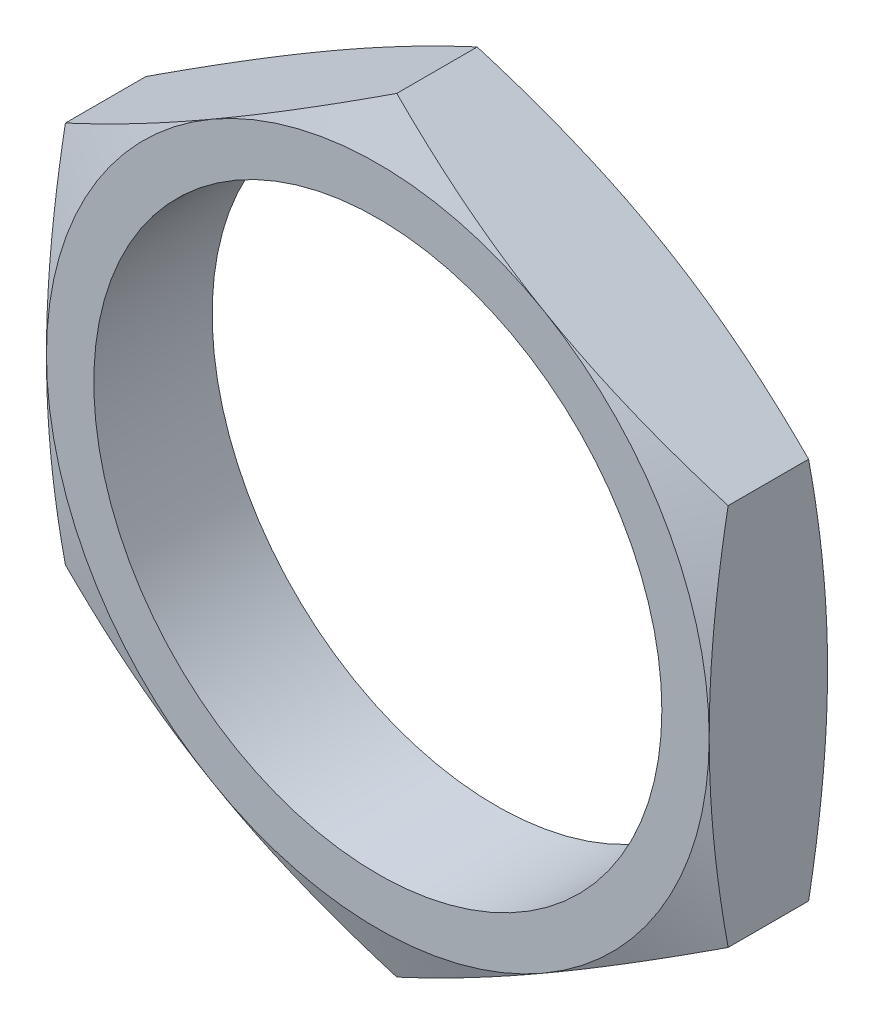
from build123d import *

# Parameters (mm, degrees)
SKETCH1_R           = 6
BOSS_EXTRUDE1_DEPTH = 2.5


with BuildPart() as part:
    # Sketch1 → Boss-Extrude1 (new body)
    with BuildSketch(Plane.XY):
        Polygon((0, 8.082903769), (-7, 4.041451884), (-7, -4.041451884), (0, -8.082903769), (7, -4.041451884), (7, 4.041451884), align=None)
        Circle(SKETCH1_R, mode=Mode.SUBTRACT)
    extrude(amount=BOSS_EXTRUDE1_DEPTH)

    # Sketch3 → Cut-Revolve1 (revolve, cut)
    with BuildSketch(Plane(origin=(0, 0, 0), x_dir=(0, 0, -1), z_dir=(1, 0, 0))):
        Polygon((-2.5, 8.082903769), (-2.1, 8.082903769), (-2.5, 7), align=None)
        Polygon((0, 8.082903769), (-0.4, 8.082903769), (0, 7), align=None)
    revolve(axis=Axis((0, 0, 0), (0, 0, 1)), mode=Mode.SUBTRACT)


solid = part.part
